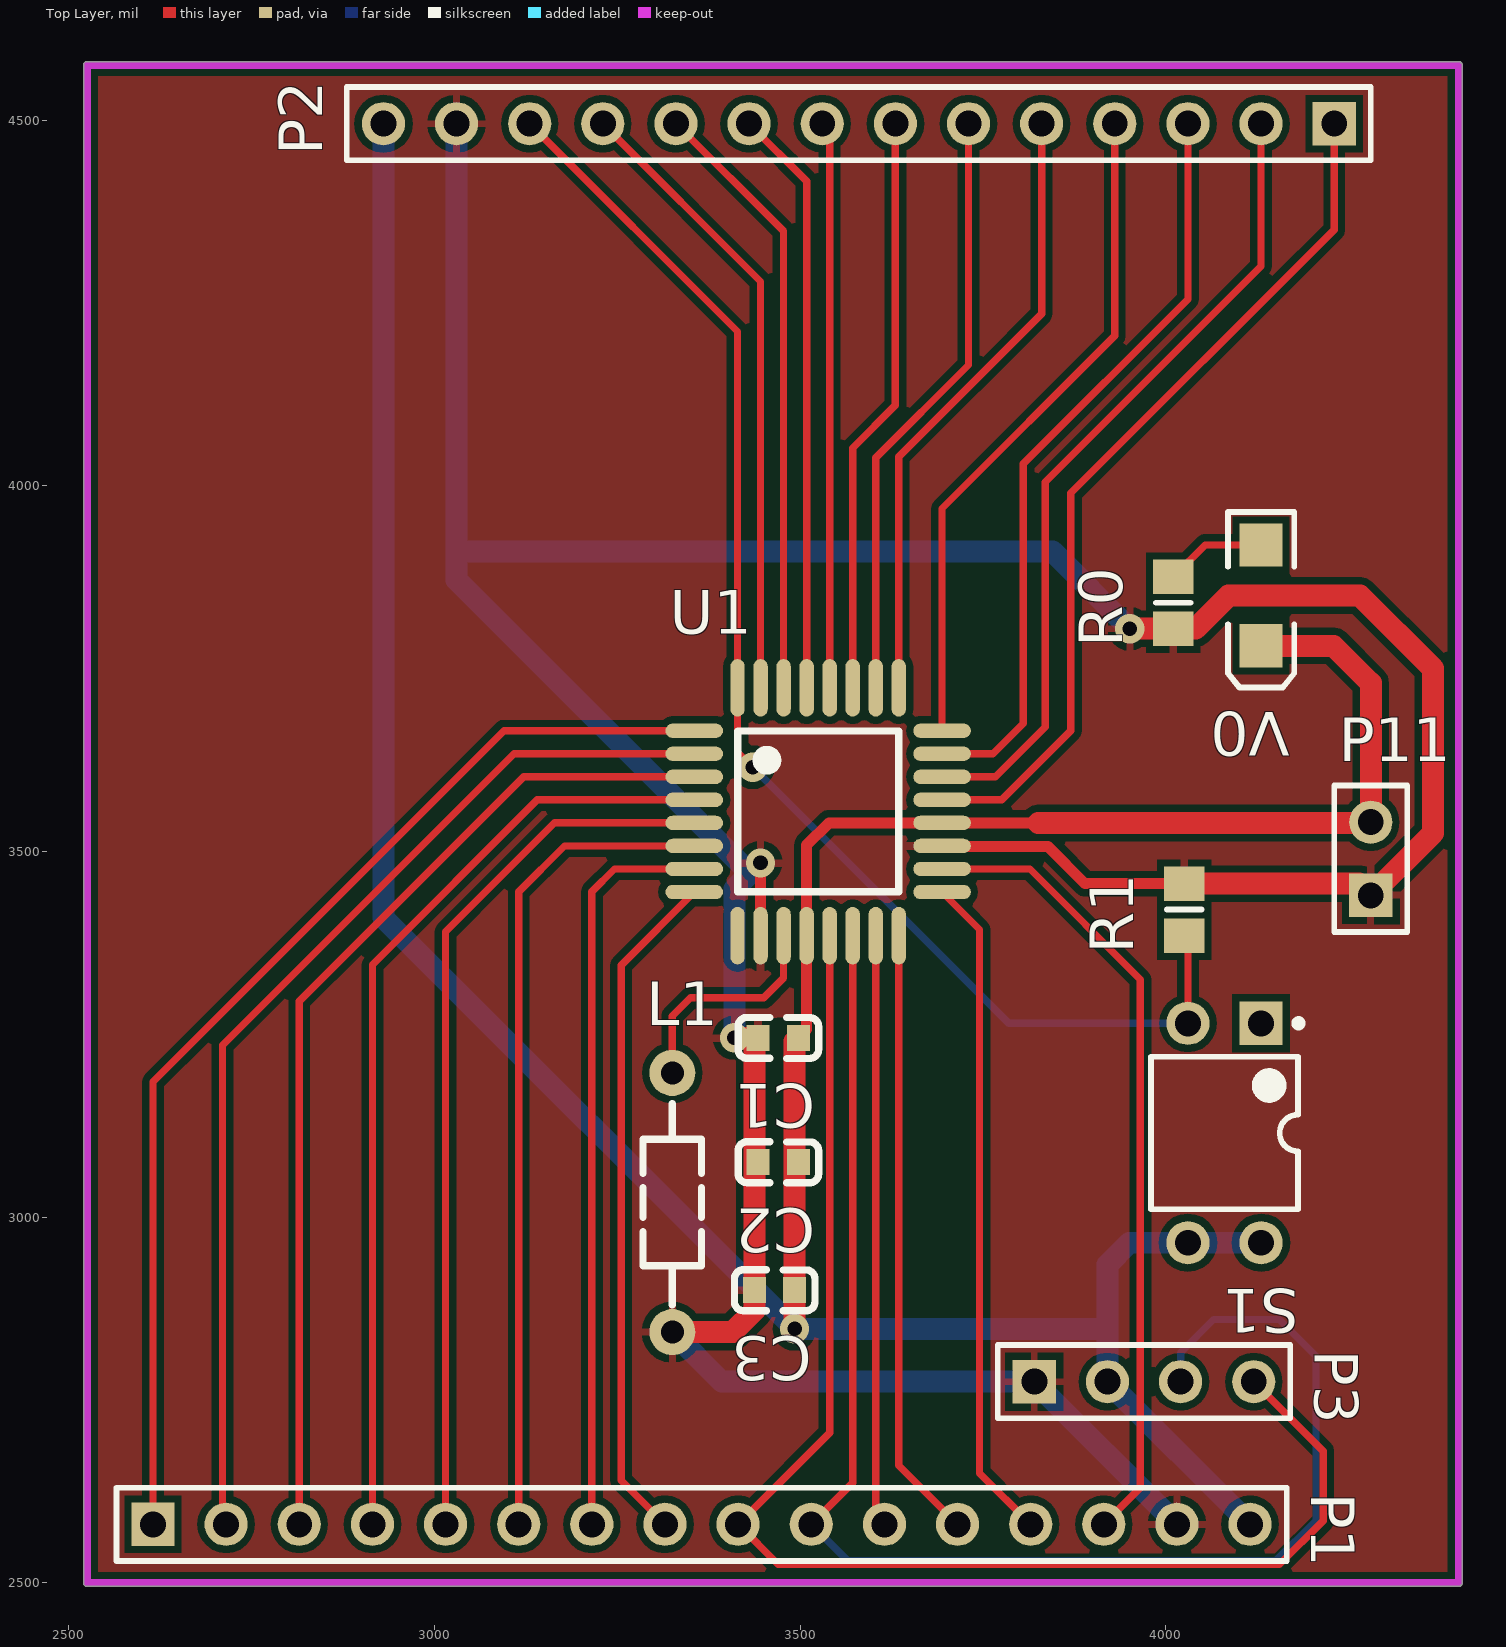
[diagram p0: Top Layer view]
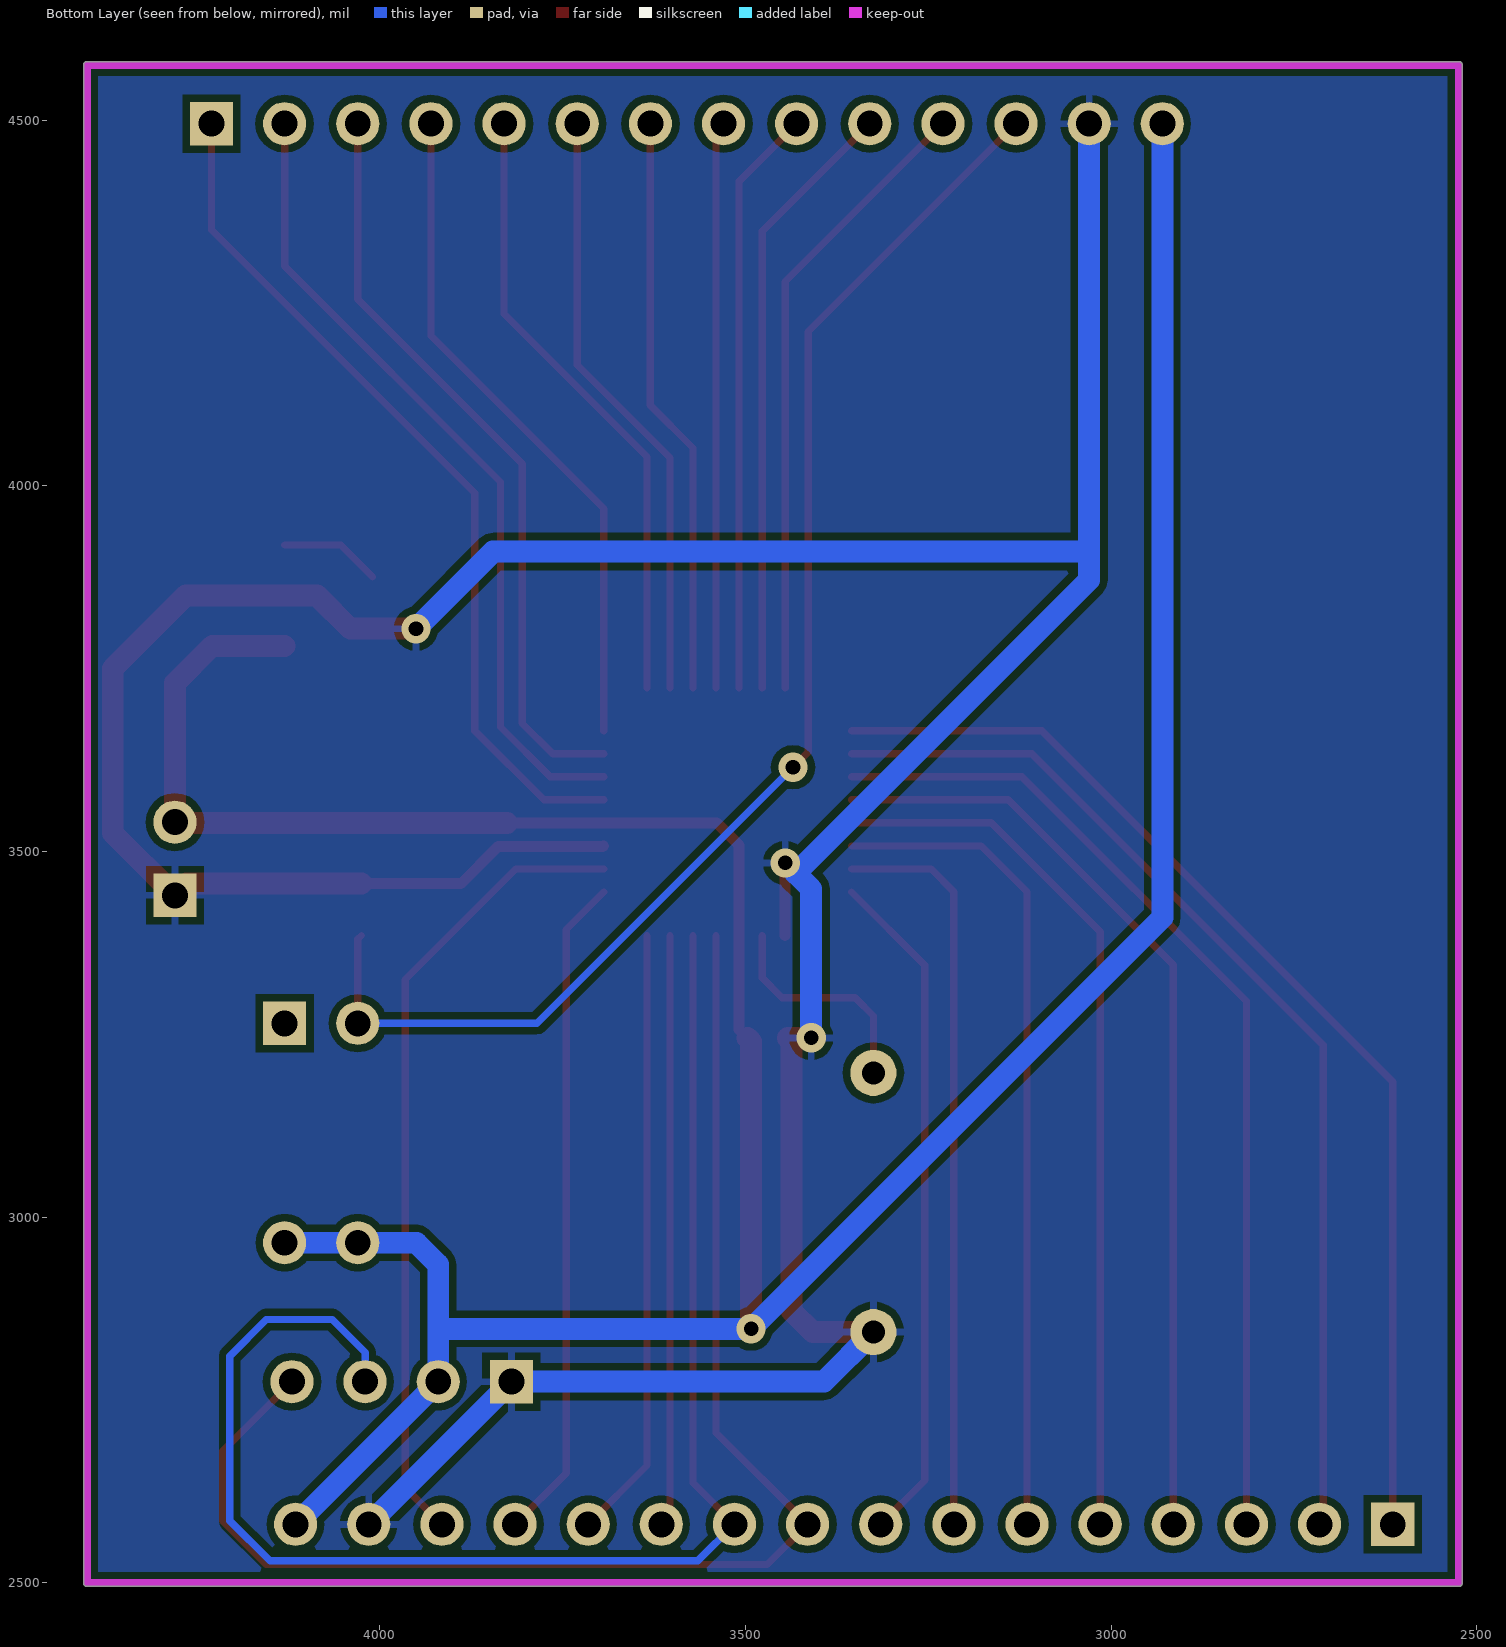
[diagram p1: Bottom Layer view, seen from below]
# Altium PCB MISC80837.PcbDoc
Units mil, origin at the board's own origin, x right, y up, seen from the top; angles counter-clockwise.
Board outline 1885.03 x 2085.03 mil, 2 copper layers (Top Layer, Bottom Layer); 13 components, 32 nets, 86 pads, 5 vias.

## Layer stack, top to bottom (the 12.6 mil dielectric is the usual default, probably not edited)
Top Solder: solder mask 0.4, Solder Resist, Dk 3.5
Top Layer: signal copper 1.4
Dielectric 1: dielectric 12.6, FR-4, Dk 4.8
Bottom Layer: signal copper 1.4
Bottom Solder: solder mask 0.4, Solder Resist, Dk 3.5

## Board outline
2519.99,2500 ccw(c2525,2500) 2525,2494.99 4400,2494.99 ccw(c4400,2500) 4405.02,2500 4405.02,4575 ccw(c4400,4575) 4400,4580.02 2525,4580.02 ccw(c2525,4575) 2519.99,4575

## Design rules (kind name [scope] priority, off if disabled: settings)
Clearance [All] p1: gap=10
MinimumSolderMaskSliver [All] p1: minsoldermaskwidth=0
PolygonConnect [All] p1: connectstyle=Relief reliefconductorwidth=10 reliefentries=4 polygonreliefangle="90 Angle" airgapwidth=10
RoutingVias [All] p1: holewidth=28 width=50 viastyle="Through Hole" minholewidth=28 minwidth=50 maxholewidth=28 maxwidth=50
SilkToSilkClearance [All] p1: silktosilkclearance=0
SilkToSolderMaskClearance [IsPad] p1: minsilkscreentomaskgap=0 clearancetoexposedcopper=TRUE
SolderMaskExpansion [All] p1: expansion=4
Width [All] p1: maxlimit=30 minlimit=10 preferedwidth=10
27 further rules are at their usual default settings.

## Components (designator, comment, footprint, x,y, rotation, side; value= is the part's Value field where it differs from the comment)
C1 "100nF" C0603 3470,3245 r180 top
C2 "100nF" C0603 3470,3075 r180 top
C3 "22uF" C0603 3465,2900 r180 top
L1 "GZ1608D601TF" AL0204 3325,3020 r90 top
P1 "Header 16" HDR1X16 2615,2580 r0 top
P2 "Header 14" HDR1X14 4230,4495 r180 top
P3 "Right-angle pin header-4P" HDR1X4 3820,2775 r0 top
P11 "HX25003-2WAG" HDR1X2 4280,3440 r90 top
R0 "10K" 6-0805_N 4010,3840 r90 top
R1 "10k" 6-0805_N 4025,3420.43 r90 top
S1 "DIP switch-2P" DIP-4 4080,3115 r270 top
U1 "STC15F2K60S2_QFP32" LQFP32 3355,3665 r0 top
V0 "Red LED_0603" 3.2X1.6X1.1 4130,3850 r270 top

## Footprints (in the part's own frame and the unit in brackets; to place one, negate y for a bottom-side part, rotate by r counter-clockwise, add the part's x,y. Pads: shape width x height; smd on the part's side, far side on the other; paste and mask are expansions set on the pad)
3.2X1.6X1.1 [mm] "SMT LED; 2 Flat Leads"
  rect 1.5x1.5 smd: 1(-1.75,0) 2(1.75,0)
  silkscreen extent -2.9,-1.15 3.2,1.15
6-0805_N [mm] "Chip Resistor, Body 2.0x1.2mm, IPC Medium Density"
  rect 1.2x1.4 smd: 1(-0.9,0) 2(0.9,0)
  silkscreen extent 0,-0.6 0,0.6, body extent -1.07,-0.7 1.07,0.7, height 0.7
AL0204 [mm] "9*2*4mm（脚距，直径，长度）"
  round 1.6 hole 0.8: 1(-4.5,0) 2(4.5,0)
  silkscreen extent -3.56,-1.02 3.43,1.02, body extent -4.75,-1.02 4.75,1.02, height 2.07
C0603 [mm]
  rect 0.8x0.9 smd paste+0 mask+0.051: 1(-0.692,-0.003) 2(0.708,-0.003)
  silkscreen extent -1.4,-0.71 1.4,0.71
DIP-4 [mm] "DIP; 4 Leads; Row Spacing 7.62 mm; Pitch 2.54 mm"
  rect 1.5x1.5 hole 0.9: 1(-3.81,1.27)
  round 1.5 hole 0.9: 2(-3.81,-1.27) 3(3.81,-1.27) 4(3.81,1.27)
  silkscreen extent -3.93,-2.55 2.65,2.7, body extent -3.15,-2.5 3.15,2.5, height 5.6
HDR1X2 [mm] "Connector; Header; 2 Position"
  rect 1.5x1.5 hole 0.9: 1(0,0)
  round 1.5 hole 0.9: 2(2.54,0)
  silkscreen extent -1.27,-1.27 3.81,1.27
HDR1X4 [mm] "Connector; Header; 4 Position"
  rect 1.5x1.5 hole 0.9: 1(0,0)
  round 1.5 hole 0.9: 2(2.54,0) 3(5.08,0) 4(7.62,0)
  silkscreen extent -1.27,-1.27 8.89,1.27
HDR1X14 [mm] "Connector; Header; 14 Position"
  rect 1.5x1.5 hole 0.9: 1(0,0)
  round 1.5 hole 0.9: 2(2.54,0) 3(5.08,0) 4(7.62,0) 5(10.16,0) 6(12.7,0) 7(15.24,0) 8(17.78,0) 9(20.32,0) 10(22.86,0) 11(25.4,0) 12(27.94,0) 13(30.48,0) 14(33.02,0)
  silkscreen extent -1.27,-1.27 34.29,1.27
HDR1X16 [mm] "Connector; Header; 16 Position"
  rect 1.5x1.5 hole 0.9: 1(0,0)
  round 1.5 hole 0.9: 2(2.54,0) 3(5.08,0) 4(7.62,0) 5(10.16,0) 6(12.7,0) 7(15.24,0) 8(17.78,0) 9(20.32,0) 10(22.86,0) 11(25.4,0) 12(27.94,0) 13(30.48,0) 14(33.02,0) 15(35.56,0) 16(38.1,0)
  silkscreen extent -1.27,-1.27 39.37,1.27
LQFP32 [mm]
  oval 2x0.5 smd: 1(0,0) 2(0,-0.8) 3(0,-1.6) 4(0,-2.4) 5(0,-3.2) 6(0,-4) 7(0,-4.8) 8(0,-5.6) 17(8.606,-5.6) 18(8.606,-4.8) 19(8.606,-4) 20(8.606,-3.2) 21(8.606,-2.4) 22(8.606,-1.6) 23(8.606,-0.8) 24(8.606,0)
  oval 0.5x2 smd: 9(1.503,-7.117) 10(2.303,-7.117) 11(3.103,-7.117) 12(3.903,-7.117) 13(4.703,-7.117) 14(5.503,-7.117) 15(6.303,-7.117) 16(7.103,-7.117) 25(7.103,1.489) 26(6.303,1.489) 27(5.503,1.489) 28(4.703,1.489) 29(3.903,1.489) 30(3.103,1.489) 31(2.303,1.489) 32(1.503,1.489)
  silkscreen extent 1.51,-5.59 7.1,-0.01, body extent -0.19,-7.33 8.81,1.67, height 1.63

## Part data
C1 C2 C3: library part CAP, "Non-polarized capacitor"
L1: library part INDUCTOR, "INDUCTOR"
P1: "Header, 16-Pin"
P2: "Header, 14-Pin"
P3: library part "Header 4", "Header, 4-Pin"
P11: library part "Header 2H", "Header, 2-Pin, Right Angle"
R0 R1: library part RES
S1: library part "SW DIP-2", "DIP Switch, 2 Position, SPST"
V0: library part LED1, "Typical RED GaAs LED"

## Via types
v1: diameter 40, hole 20, Top Layer to Bottom Layer, 5 vias

## Nets (pads, with @x,y where several pads share a name; then routed paths per layer and width w, separated by ;. In a path a pad name is that pad's centre, name@x,y a point inside that pad or via, vN(x,y) a via of type N, cw(c..) or ccw(c..) an arc to the next point about the centre after c; other vN are vias at no path point)
DEBUG_RX: P1.9 P3.4 U1.13 | length 1933.6
  Top Layer w10: U1.13 3540.17,2705.17 P1.9 3470,2525 4155,2525 4215,2585 4215,2680 P3.4
DEBUG_TX: P1.10 P3.3 U1.14 | length 2051.1
  Top Layer w10: P1.10 3571.66,2636.66 U1.14
  Bottom Layer w10: P1.10 3565,2530 4150,2530 4205,2585 4205,2810 4155,2860 4065,2860 4020,2815 P3.3
"MOD SET": S1.1
NetL1_2: L1.2 U1.11 | length 309.2
  Top Layer w10: L1.2 3325,3275 3350,3300 3450,3300 3477.17,3327.17 U1.11
NetR0_2: R0.2 V0.1 | length 138
  Top Layer w10: R0.2 4053.46,3918.9 V0.1
"OORIGIN ID": P2.12 R1.1 S1.2 U1.32 | length 1868.4
  Top Layer w10: P2.12 3414.18,4210.82 U1.32 3414.18,3635.82 v1(3435,3615) ; R1.1 4030,3380 S1.2
  Bottom Layer w10: v1(3435,3615) 3785,3265 S1.2
P0.0: P2.9 U1.29 | length 804
  Top Layer w10: P2.9 3508.67,4416.33 U1.29
P0.1: P2.10 U1.30 | length 832.3
  Top Layer w10: P2.10 3477.17,4347.83 U1.30
P0.2: P2.11 U1.31 | length 860.7
  Top Layer w10: P2.11 3445.68,4279.32 U1.31
P1.0: P1.1 U1.1 | length 1543.8
  Top Layer w10: P1.1 2615,3185 3095,3665 U1.1
P1.1: P1.2 U1.2 | length 1467.1
  Top Layer w10: P1.2 2710,2585 2710,3235 3108.5,3633.5 U1.2
P1.2: P1.3 U1.3 | length 1382.2
  Top Layer w10: P1.3 2815,3295 3122.01,3602.01 U1.3
P1.3: P1.4 U1.4 | length 1298.4
  Top Layer w10: P1.4 2915,3345 3140.51,3570.51 U1.4
P1.4: P1.5 U1.5 | length 1211.7
  Top Layer w10: P1.5 3015,3390 3164.02,3539.02 U1.5
P1.5: P1.6 U1.6 | length 1130.9
  Top Layer w10: P1.6 3115,3445 3177.52,3507.52 U1.6
P1.6: P1.7 U1.7 | length 1017.9
  Top Layer w10: P1.7 3215,3445 3246.02,3476.02 U1.7
P1.7: P1.8 U1.8 | length 930.8
  Top Layer w10: P1.8 3255,2640 3255,3344.53 U1.8
P2.0: P2.1 U1.21 | length 1194.4
  Top Layer w10: U1.21 3775.51,3570.51 3870,3665 3870,3990 4230,4350 P2.1
P2.1: P2.2 U1.22 | length 1116.5
  Top Layer w10: U1.22 3767.01,3602.01 3835,3670 3835,4005 4130,4300 P2.2
P2.2: P2.3 U1.23 | length 1041.6
  Top Layer w10: U1.23 3763.5,3633.5 3805,3675 3805,4030 4030,4255 P2.3
P2.3: P2.4 U1.24 | length 927.8
  Top Layer w10: U1.24 3693.83,3968.83 3930,4205 P2.4
P2.4: P2.5 U1.25 | length 852.3
  Top Layer w10: U1.25 3634.65,4039.65 3830,4235 P2.5
P2.5: P2.6 U1.26 | length 823.9
  Top Layer w10: U1.26 3603.16,4038.16 3730,4165 P2.6
P2.6: P2.7 U1.27 | length 795.5
  Top Layer w10: U1.27 3571.66,4051.66 3630,4110 P2.7
P2.7: P2.8 U1.28 | length 775.6
  Top Layer w10: P2.8 3540.17,4484.83 U1.28
P3.2: P1.11 U1.15 | length 809.7
  Top Layer w10: U1.15 3603.16,2591.84 P1.11
P3.3: P1.12 U1.16 | length 838.1
  Top Layer w10: U1.16 3634.65,2660.35 P1.12
P3.4: P1.13 U1.17 | length 914.7
  Top Layer w10: U1.17 3745,3393.36 3745,2650 P1.13
P3.5: P1.14 U1.18 | length 1099.4
  Top Layer w10: U1.18 3813.98,3476.02 3965,3325 3965,2630 P1.14
P3.6: C1.2 C2.2 C3.2 L1.1 P1.15 P2.13 P3.1 P11.1 R0.1 R1.2 U1.10 U1.19 | length 5253.1
  Top Layer w15: U1.10 v1(3445.68,3484.32) ; U1.19 3694.84,3506.52 3838.48,3506.52 3889.13,3455.87 R1.2
  Top Layer w30: L1.1 3407.83,2842.83 3437.14,2872.14 C3.2 3437.14,3240.11 C1.2 v1(3410.11,3245.11) v1@3410,3245 ; v1(3950.43,3804.57) R0.1 4040.32,3804.57 4085.75,3850 4265,3850 4365,3750 4365,3525 P11.1 4264.13,3455.87 R1.2
  Bottom Layer w30: P2.13 3030,3910 ; L1.1 3392.83,2775 P3.1 P1.15 ; v1(3410.11,3245.11) 3410.11,3448.75 3431.35,3470 3030,3871.35 3030,3910 ; v1(3950.43,3804.57) 3845,3910 3030,3910
P3.7: C1.1 C2.1 C3.1 P1.16 P2.14 P3.2 P11.2 S1.3 S1.4 U1.12 U1.20 V0.2 | length 4783.5
  Top Layer w15: C1.1 3508.67,3256.53 U1.12 3508.67,3508.67 3539.02,3539.02 U1.20 3825.98,3539.02
  Top Layer w30: v1(3492.25,2847.25) C3.1 3492.25,3240.11 C1.1 ; 3825.98,3539.02 4279.02,3539.02 P11.2 4280,3730 4228.9,3781.1 V0.2
  Bottom Layer w30: P2.14 2930,3409.49 v1(3492.25,2847.25) 3912.25,2847.25 3920,2855 ; P1.16 P3.2 3920,2855 ; S1.4 S1.3 3950,2965 3920,2935 3920,2855
RST: U1.9

## Polygon pours and split planes (outlines as drawn)
P3.6 on Bottom Layer "G" (solid, remove dead copper, pour order 0): 1945,4810 2045,4710 4875,4710 4875,2505 4530,2160 4385,2305 1740,2305
P3.6 on Top Layer "G" (solid, remove dead copper, pour order 2): 2310,4705 4865,4705 4945,4625 4610,4290 4610,2145 2195,2145 2115,2225

## Keep-outs
Keep-Out Layer:
  lines w10: 2805,4575 4400,4575 4400,2500 2575,2500 2525,2500 2525,4575 2855,4575